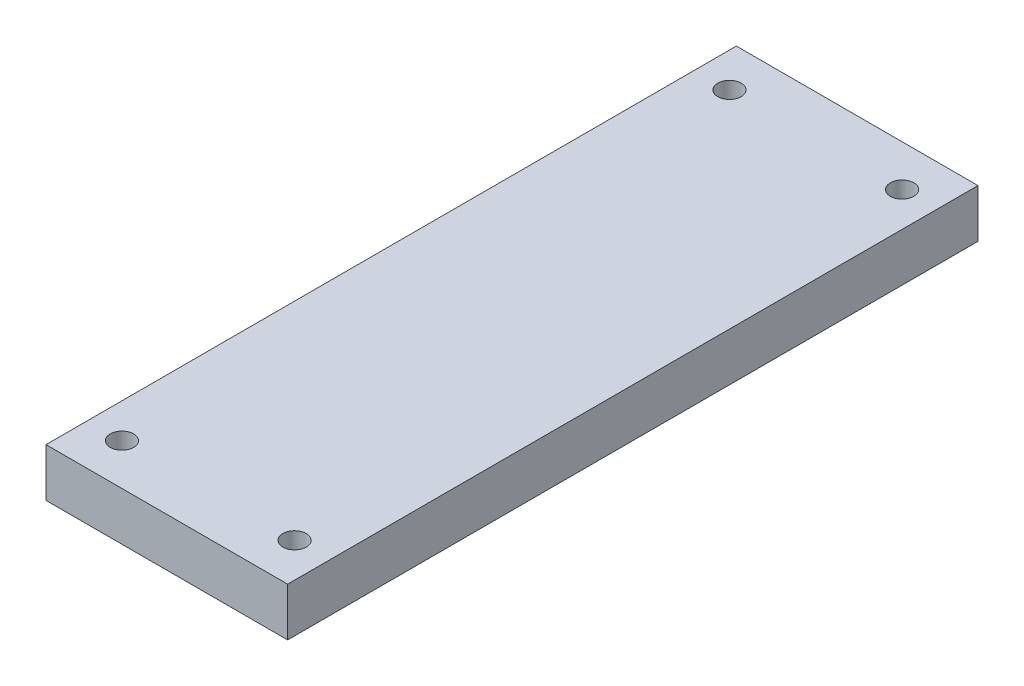
from build123d import *

# Parameters (mm, degrees)
SKETCH1_W           = 70
SKETCH1_H           = 200
BOSS_EXTRUDE1_DEPTH = 14
M8_TAPPED_HOLE1_D   = 6.8


with BuildPart() as part:
    # Sketch1 → Boss-Extrude1 (new body)
    with BuildSketch(Plane(origin=(0, 0, 0), x_dir=(1, 0, 0), z_dir=(0, 1, 0))):
        with Locations((35, 100)):
            Rectangle(SKETCH1_W, SKETCH1_H)
    extrude(amount=BOSS_EXTRUDE1_DEPTH)

    # M8 Tapped Hole1 (through all)
    with Locations(Plane(origin=(0, 0, 0), x_dir=(-1, 0, 0), z_dir=(0, -1, 0))):
        with Locations((-60, 188), (-10, 188), (-10, 12), (-60, 12)):
            Hole(M8_TAPPED_HOLE1_D / 2)


solid = part.part
